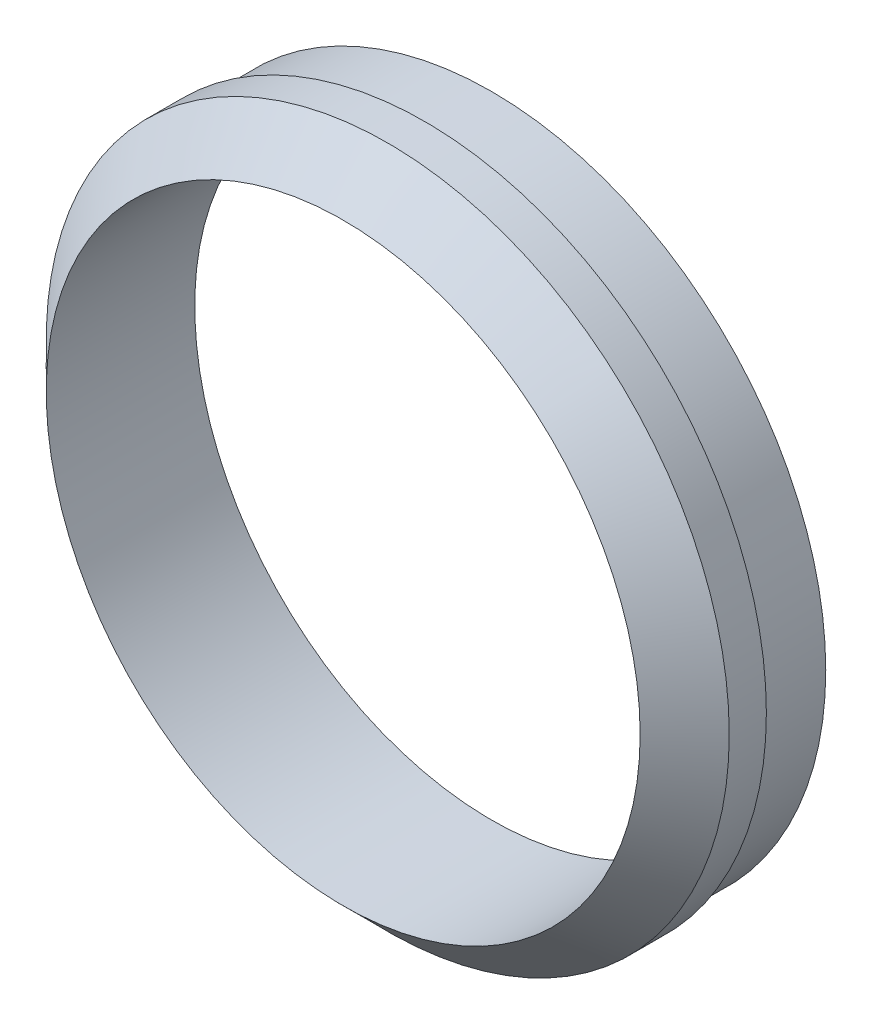
from build123d import *


with BuildPart() as part:
    # Sketch1 → Revolve1 (revolve)
    with BuildSketch(Plane(origin=(0, 0, 0), x_dir=(1, 0, 0), z_dir=(0, 1, 0))):
        Polygon((8, 4), (8, 0), (9.2, 1.2), (9.2, 2.2), (9, 2.2), (9, 4), align=None)
    revolve(axis=Axis((0, 0, -4), (0, 0, 1)))


solid = part.part
